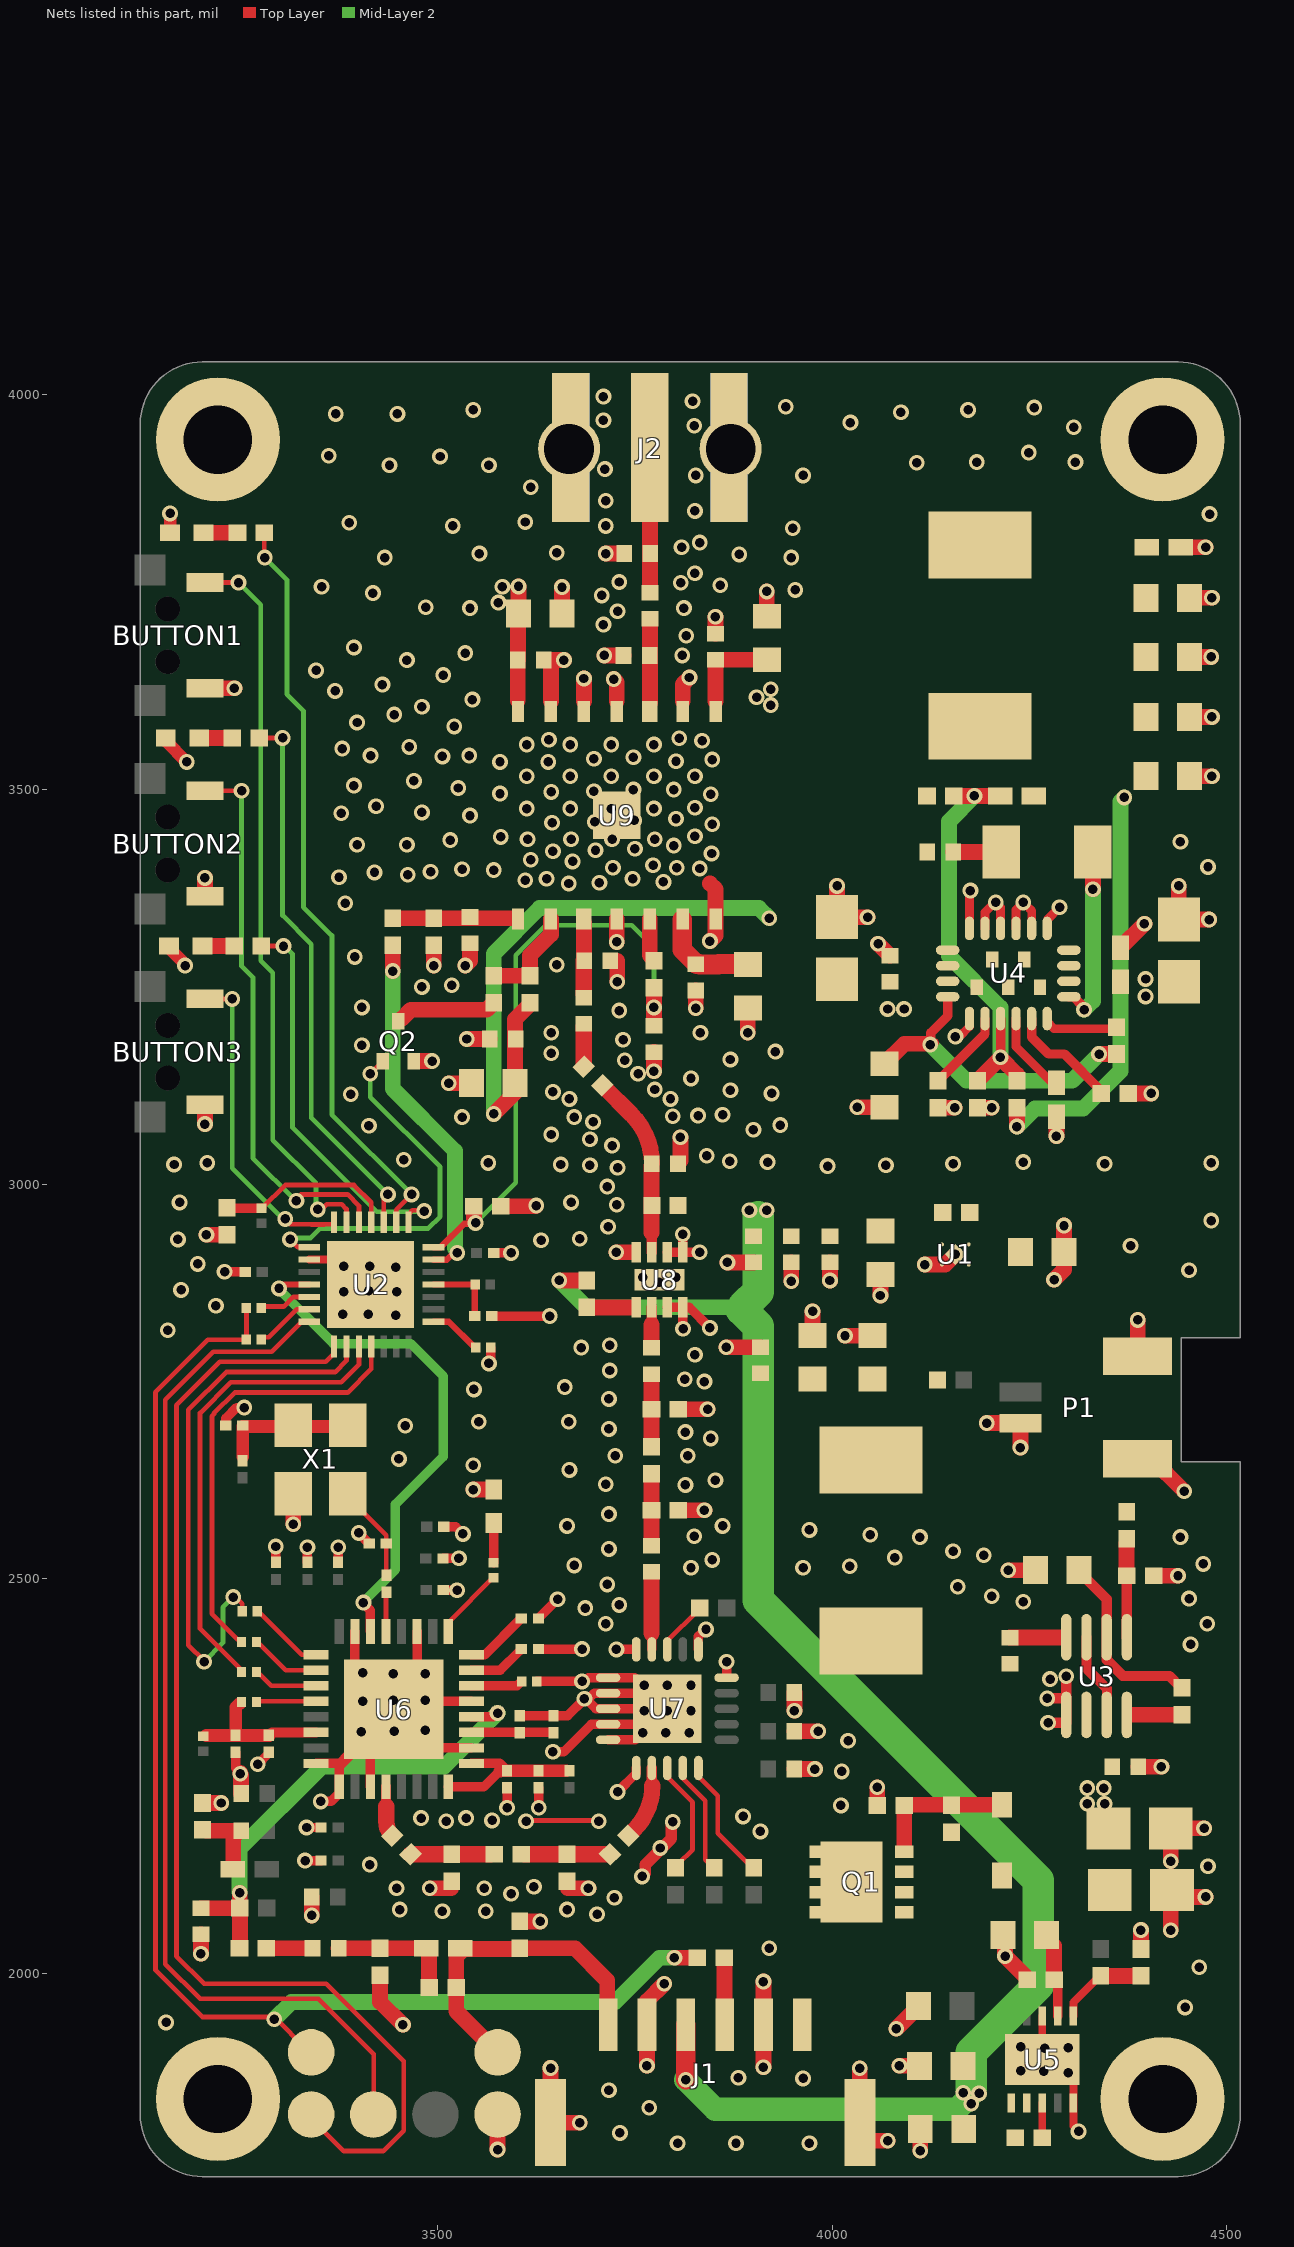
[diagram p0: the nets of this part, all layers, seen from the top]
# Altium PCB MISC79034.PcbDoc (part 2 of 2)
Units mil, origin at the board's own origin, x right, y up, seen from the top; angles counter-clockwise.
Board outline 1393.7 x 2299.21 mil, 4 copper layers (Top Layer, Mid-Layer 1, Mid-Layer 2, Bottom Layer); 179 components, 97 nets, 521 pads, 554 vias.

## Via types
v1: diameter 20, hole 12, Top Layer to Bottom Layer, tented both sides, 554 vias

## Nets (pads, with @x,y where several pads share a name; then routed paths per layer and width w, separated by ;. In a path a pad name is that pad's centre, name@x,y a point inside that pad or via, vN(x,y) a via of type N, cw(c..) or ccw(c..) an arc to the next point about the centre after c; other vN are vias at no path point) (continued)
GND: BUTTON1.1 BUTTON2.1 BUTTON3.1 C1.2 C2.2 C3.2 C4.2 C5.1 C7.1 C8.2 C9.2 C10.2 C11.2 C12.2 C13.2 C14.2 C15.2 C16.2 C17.2 C18.2 C19.1 C20.2 C21.2 C22.1 C23.1 C24.1 C25.1 C26.2 C28.1 C29.2 C30.2 C31.1 C32.1 C33.1 C34.1 C35.2 C36.2 C37.1 C38.2 C39.1 C47.2 C50.2 C51.1 C52.2 C53.1 C54.2 C55.2 C56.1 C57.1 C58.1 C59.1 C60.1 C61.1 C62.1 C63.1 C64.2 C65.2 C67.2 C68.1 C70.1 C71.1 C72.1 C73.2 C74.2 C75.2 C76.2 C78.2 C80.1 C82.2 C83.2 C84.2 J1.2 J1.5 J1.7 J1.8 J2.2 LED1.2 LED2.2 LED3.2 LED4.2 P1.1 P1.3 P1.4 P2.1 Q2.2 R3.1 R6.1 R13.2 R14.2 R15.2 R21.2 R25.1 R29.2 R31.2 R32.2 R33.2 R45.2 R51.2 R52.2 R53.2 R56.2 R57.1 SCREW1.1 SCREW2.1 SCREW3.1 SCREW4.1 SR1.2 U1.2 U1.5 U2.16 U2.29 U3.5 U4.1 U4.11 U4.12 U4.13 U4.14 U4.15 U4.16 U5.5 U5.8 U5.11 U6.8 U6.9 U6.11 U6.18 U6.21 U6.27 U6.31 U6.33 U7.1 U7.10 U7.11 U7.15 U7.16 U7.17 U7.18 U7.19 U7.20 U7.21 U8.3 U8.4 U8.5 U8.6 U8.8 U8.9 U9.4 U9.7 U9.9 U9.11 U9.12 U9.13 U9.15 X1.2 | length 5669
  Top Layer w6: v1@3614,2194 v1@3704,2194
  Top Layer w10: U2.16@3337.26,2904.5 U2.29@3363.5,2904.5 ; U5.11@4266,1921 U5.8@4266,1946.12 ; U5.11@4305.4,1860.4 U5.5@4305.4,1835.88 4305.4,1806.6 v1(4312,1800)
  Top Layer w11: v1(4156,3187) 4161,3187 4173.79,3199.79 U4.1@4173.79,3209.91 ; U4.16@4173.79,3324.09 4173.79,3372 v1(4175,3372) ; U4.15@4193.47,3324.09 4193.47,3344.47 v1@4202,3353 ; v1(4207,3357) 4213.16,3350.84 U4.14@4213.16,3324.09 ; U4.13@4232.84,3324.09 4232.84,3347.84 v1(4242,3357) ; v1@4246,3353 4252.53,3346.47 U4.12@4252.53,3324.09 ; U4.11@4272.21,3324.09 4272.21,3335.21 v1(4288,3351)
  Top Layer w12: v1(3230,2889) C14.2@3256.4,2889 ; C51.1@3231.55,2694.31 3231.55,2703.31 3245.24,2717 v1(3255,2717) ; C68.1@3244,2280.2 3244,2260 v1@3250,2254 ; v1(3272,2265) 3286,2279 C67.2@3286,2280.2 ; C58.1@3295,2520.8 v1(3295,2541) ; v1(3332,2143) C53.1@3352.2,2143 ; v1(3334,2185) C52.2@3352.2,2185 ; C63.1@3335,2520.8 v1(3335,2540) ; U6.8@3346,2266.1 3376.1,2266.1 U6.33@3386,2276 ; v1(3352,2218) 3365,2218 3375.52,2228.52 U6.9@3375.52,2236.58 3375.52,2262.52 3393,2280 U6.33@3398,2280 ; C64.2@3374,2520.8 v1(3374,2540) ; U6.33@3395.21,2390.21 U6.31@3395.21,2433.42 ; v1(3400,2558.2) C47.2@3413.2,2545 ; U6.11@3414.89,2236.58 U6.33@3414.89,2274.89 ; U6.33@3473.95,2391.95 U6.27@3473.95,2433.42 ; U6.33@3503.16,2344.84 U6.21@3542.84,2344.84 ; U6.33@3504.21,2285.79 U6.18@3542.84,2285.79 ; C37.1@3506.8,2526 v1(3527,2526) ; C38.2@3507.26,2485.62 v1(3524.62,2485.62) ; C39.1@3507.8,2566 3523,2566 v1(3532,2557) ; v1(3565,2773) 3567.51,2775.51 R6.1@3567.51,2793 ; C7.1@3568.8,2833 v1(3642,2833) ; C16.2@3570.8,2913 v1(3593,2913) ; v1(3588,2210) C36.2@3588,2235.2 ; C30.2@3604,2326.8 C28.1@3647,2326.8 3664.8,2326.8 v1(3686,2348) ; R25.1@3625.51,2370 v1(3683,2370) ; C29.2@3627.8,2411 v1(3683,2411) ; C32.1@3627.8,2450 v1(3652,2474.2) ; v1(3628,2210) C34.1@3628,2235.2 ; v1(3646,2281) 3660,2281 3694.78,2315.78 U7.19@3715.9,2315.78 U7.21@3749.78,2315.78 ; v1@3687,2371 3690.83,2374.83 U7.16@3715.9,2374.83 3749.83,2374.83 U7.21@3750,2375 ; v1@3691,2345 3700.54,2335.46 U7.18@3715.9,2335.46 U7.21@3750.54,2335.46 ; v1@3693,2350 3698.15,2355.15 U7.17@3715.9,2355.15 U7.21@3750.15,2355.15 ; U7.20@3715.9,2296.09 U7.21@3750.09,2296.09 ; v1(3726.44,2410.56) U7.15@3749,2410.56 ; v1(3728,2230) 3751.63,2253.63 U7.1@3751.63,2260.36 ; U8.3@3790.84,2844.16 3818.84,2844.16 v1(3845,2818) ; U8.6@3790.84,2913.84 v1(3831.84,2913.84) ; U8.4@3810.53,2844.16 3810.53,2817.47 v1(3811,2817) ; U8.5@3810.53,2913.84 v1(3810.53,2936.53) ; U7.11@3830.37,2410.56 3830.37,2427.37 3840,2437 v1(3840,2436) ; U7.10@3866.1,2376 v1(3866.1,2394.9)
  Top Layer w13: v1(4272.41,2348.59) 4296.41,2348.59 U3.5@4296.41,2327.58 ; v1(4273.41,2317.59) 4296.41,2317.59 U3.5@4296.41,2327.58 ; v1(4296.41,2376.59) U3.5@4296.41,2327.58
  Top Layer w15: v1(3759,2123) 3763,2127 3763,2138 3796,2171 v1@3796,2189
  Top Layer w16: LED1.2@3155.61,3565.47 3155.61,3561.39 v1(3182,3535) ; LED3.2@3159.55,3301.69 3159.55,3299.45 3181,3278 v1(3180,3277) ; LED2.2@3161.05,3825.31 v1(3161.05,3849.95)
  Top Layer w20: v1(3200,2025) C80.1@3200,2049.46 ; R53.2@3202,2216.04 v1(3225.96,2216.04) ; v1(3205.14,3076.14) BUTTON3.1@3205.14,3100.9 ; BUTTON2.1@3205.14,3364.68 v1(3205.14,3388.14) ; BUTTON1.1@3205.14,3628.46 v1(3242.54,3628.46) ; v1(3207.04,2935.96) SR1.2@3233,2935.96 ; v1(3250,2253) v1@3250,2254 ; C78.2@3250.88,2228 v1@3250.88,2250.88 ; v1(3317.1,2569.1) X1.2@3317.1,2608 ; v1(3340.46,2073.54) C59.1@3340.46,2097 ; R51.2@3427,1997.96 3427,1964 v1(3456,1935) ; Q2.2@3475,3156 v1@3492,3156 ; v1(3490.04,2107.96) R31.2@3517,2107.96 ; v1(3495,3277) R45.2@3495,3302.96 ; v1(3514,3128) C56.1@3542.9,3128 ; v1(3535,3277) 3541,3283 C5.1@3541,3304.46 ; v1(3537,3184) C57.1@3565.92,3184 ; v1(3545.19,2613.19) LED4.2@3571,2613.19 ; v1(3575.94,1776.94) P2.1@3575.94,1821.38 ; R21.2@3580.04,2972 v1@3624,2972 ; R52.2@3604,2066.04 v1(3629.96,2066.04) ; C54.2@3634.54,3664 v1(3660,3664) ; v1(3643.12,1880.12) J1.8@3643.12,1810.98 v1(3679.98,1810.98) ; U9.13@3643.54,3611.8 C54.2@3643.54,3658.46 ; C55.2@3657.56,3723 v1(3657.56,3756.56) ; R32.2@3665,2107.96 v1(3691.04,2107.96) ; U9.12@3685.27,3611.8 v1(3685.27,3640.73) ; v1(3711,3670) C71.1@3735.46,3670 ; v1(3713,3799) C72.1@3736.46,3799 ; v1(3723,3640) 3727,3636 U9.11@3727,3611.8 ; v1(3726.16,2913.84) U8.8@3746,2913.84 ; v1(3727,3307) U9.4@3727,3336.2 ; v1(3727.54,3256.54) C65.2@3727.54,3283 ; v1(3765.16,1883.16) J1.2@3765.16,1935 3765.16,1965.16 v1(3787,1987) ; v1(3774,3143) C70.1@3774,3167.46 ; C50.2@3807.54,3030 v1(3807.54,3059.54) ; U9.9@3810.46,3611.8 3810.46,3633.46 v1(3819,3642) ; R29.2@3813.04,2587 v1(3838,2587) ; R33.2@3814.04,2715 v1(3842,2715) ; v1(3827,3223) C74.2@3827,3245.46 ; v1(3845,3308) 3852.2,3315.2 U9.7@3852.2,3336.2 3852.2,3373.8 3845,3381 ; C76.2@3852,3697.54 v1(3852,3719) ; v1(3865.54,2793.54) C13.2@3909,2793.54 ; v1(3867.08,2900.92) C33.1@3900,2900.92 ; v1(3893,3192) C73.2@3893,3223.44 ; v1(3912.81,1881.19) J1.5@3912.81,1935 v1(3912.81,1989.81) ; C75.2@3917,3719.56 v1(3917,3751) ; v1(3948,2877) C31.1@3948,2900.92 ; C61.1@3952,2259 v1(3978,2259) ; C60.1@3952,2307 v1(3982,2307) ; v1(3952,2333) C62.1@3952,2356 ; C12.2@3975,2808.56 v1(3975,2839) ; v1(3997,2878) C35.2@3997,2900.92 ; v1(4006,3378) C2.2@4006,3338.37 v1(4044.63,3338.37) ; v1(4016.12,2808.12) C11.2@4051,2808.12 ; v1(4031.56,3097.44) C84.2@4066,3097.44 ; v1(4034.85,1879.85) J1.7@4034.85,1810.98 4034.85,1788.15 v1(4070.15,1788.15) ; R3.1@4056.96,2213 v1(4056.96,2235.96) ; v1(4058,3304.54) C17.2@4073,3289.54 ; v1(4061,2859) C3.2@4061,2885.44 ; v1(4081,1930) 4109.44,1958.44 C24.1@4109.44,1959 ; v1(4085,1883) C26.2@4110.44,1883 ; v1(4111.44,1775.56) C23.1@4111.44,1803 ; v1(4117.2,2898.2) U1.2@4139.07,2898.2 4143.2,2898.2 U1.5@4154,2909 ; R13.2@4134,3096.96 v1(4154.96,3096.96) ; R14.2@4184,3096.92 v1(4201.92,3096.92) ; v1(4195.64,2697.36) P1.1@4238.35,2697.36 v1(4238.35,2666.35) ; C25.1@4216.44,2049 4219,2046.44 v1(4219,2022) 4246.96,1994.04 R57.1@4246.96,1992 ; v1(4223,2511) C1.2@4257.44,2511 ; v1(4281,2879) 4293.56,2891.56 C4.2@4293.56,2914 v1(4293.56,2947.56) ; v1(4284,3061) C22.1@4284,3085.54 ; C18.2@4365,3299.46 v1(4395.54,3330) ; P1.4@4386.97,2652.09 4404.91,2652.09 v1@4445,2612 ; P1.3@4386.97,2782.01 v1(4387,2828) ; C8.2@4387.91,2262 v1(4417,2262) ; R56.2@4391,2031.04 v1(4391,2055) ; R15.2@4407.04,2504 v1(4438,2504) ; v1(4428.74,2054.74) 4428.74,2097 v1(4473,2097) ; v1(4428.74,2142.26) C9.2@4428.74,2184 v1(4471,2184) ; v1(4439,3378) C15.2@4439,3335.37 v1(4477.37,3335.37) ; C19.1@4441.46,3807 v1(4473,3807) ; C21.2@4452.56,3517 v1(4481,3517) ; C83.2@4452.56,3592 v1(4481,3592) ; C20.2@4452.56,3668 v1(4480,3668) ; C82.2@4452.56,3743 v1(4481,3743)
  other v1: 3804,1785 3878,1785 3971,1785 3731,1798 3768,1830 3717,1852 3963,1867 3881,1868 4299,1874 4268,1876 4239,1877 4269,1905 4299,1906 4239,1907 3156,1938 4447,1957 4465,2008 3920,2032 3702,2075 3506,2079 3561,2079 3452,2081 3664,2081 3724,2096 3593,2101 3448,2108 3559,2108 3622,2110 4476,2136 3414,2138 3782,2159 3909,2180 3798,2192 3511,2193 3612,2193 3704,2193 3569,2194 3479,2197 3536,2197 3887,2199 4011,2213 4012,2256 4020,2295 3760,2305 3789,2305 3819,2305 3403,2306 3445,2307 3484,2308 3762,2333 3791,2333 3821,2333 3405,2345 3444,2346 3484,2346 3762,2365 3791,2365 3821,2365 4276,2373 3444,2380 3484,2380 3405,2381 4454,2417 3713,2443 4475,2443 3687,2463 3730,2467 4242,2471 4452,2475 4202,2478 4159,2490 3715,2493 3821,2514 3963,2514 4022,2516 3673,2517 4470,2519 3848,2524 4079,2527 4192,2530 4153,2535 3717,2538 4111,2553 4441,2553 3825,2554 4048,2556 3971,2562 3664,2567 3861,2567 3717,2582 4446,2611 3814,2619 3713,2620 3852,2625 3667,2638 3545,2644 3451,2652 3725,2656 3817,2656 3846,2678 3814,2686 3717,2690 3459,2694 3552,2699 3666,2699 3717,2728 3546,2740 3661,2743 3838,2750 3813,2753 3718,2764 3826,2784 3682,2793 3718,2796 3158,2815 3447,2834 3380,2835 3412,2835 3219,2846 3381,2864 3448,2864 3413,2865 3175,2866 3781,2876 3760,2882 3802,2882 4452,2891 3447,2895 3381,2896 3414,2896 3196,2899 4156,2911 4378,2922 3631,2929 3171,2930 3680,2931 3716,2946 4480,2954 3625,2973 3727,2974 3173,2977 3669,2977 3715,2997 3728,3021 3994,3023 3693,3024 4068,3024 3166,3025 3656,3025 4153,3026 4345,3026 3208,3027 3564,3027 4480,3027 3918,3028 4242,3028 3870,3029 3457,3031 3841,3036 3721,3049 3693,3057 3644,3063 3900,3069 3413,3074 3934,3075 3697,3079 3531,3085 3673,3085 3798,3086 3830,3087 3861,3088 3667,3108 3795,3108 3390,3114 3923,3115 3646,3117 3871,3119 3775,3120 3821,3134 3754,3140 3493,3156 3737,3157 3871,3158 3644,3166 3928,3168 3404,3176 3735,3183 3644,3192 3833,3192 3730,3220 3404,3224 3480,3250 3518,3252 3651,3278 3395,3288 3383,3356 3666,3381 3705,3382 3786,3383 3611,3385 3638,3387 3747,3387 3375,3389 3462,3392 3420,3395 3491,3396 3571,3398 3531,3399 3832,3400 3722,3401 3803,3401 4476,3402 3773,3404 3671,3409 3618,3411 3847,3419 3646,3422 3700,3423 3750,3425 3799,3429 3398,3430 3461,3430 4441,3434 3516,3436 3614,3437 3669,3437 3721,3437 3775,3437 3580,3440 3826,3441 3848,3456 3645,3458 3699,3459 3749,3461 3802,3463 3541,3467 3378,3470 3480,3471 3613,3476 3668,3476 3720,3476 3774,3476 3826,3477 3422,3479 3846,3494 3579,3495 3644,3497 3698,3498 3748,3500 3799,3500 3526,3502 3394,3505 3470,3511 3613,3517 3668,3517 3720,3517 3774,3517 3826,3517 3579,3535 3640,3535 3802,3536 3848,3538 3698,3539 3748,3541 3506,3542 3415,3543 3540,3543 3379,3552 3464,3554 3613,3557 3668,3557 3720,3557 3774,3557 3835,3562 3641,3563 3806,3565 3521,3580 3398,3585 3445,3595 3480,3605 3544,3614 3370,3625 3430,3633 3507,3645 3346,3651 3461,3664 3810,3670 3535,3673 3394,3680 3815,3695 3710,3709 3728,3726 3541,3730 3812,3730 3485,3731 3708,3746 3418,3749 3953,3753 3353,3757 3858,3759 3808,3762 3730,3763 3826,3774 3433,3794 3948,3794 3882,3798 3553,3799 3651,3800 3809,3807 3832,3813 3950,3831 3519,3834 3713,3834 3388,3838 3611,3839 4478,3849 3826,3853 3713,3866 3618,3883 3827,3898 3963,3898 3712,3906 3439,3911 3565,3911 4107,3914 4183,3915 4308,3915 3503,3922 3362,3923 4249,3927 4306,3959 3825,3961 4023,3965 3710,3968 3371,3976 3449,3976 4087,3978 3545,3981 4172,3981 4256,3984 3941,3985 3823,3992 3710,3998
I_RC: P6.1 R4.2 R7.2 R8.2 | length 1715.7
  Top Layer w6: R7.2@3257.49,2803 3209,2803 3142.5,2736.5 3142.5,2404.5 3142.5,2004.5 3202,1945 3293,1945 P6.1@3335,1903 ; R7.2@3257.69,2804.69 R8.2@3257.69,2843
  Top Layer w20: v1(3800,2020) R4.2@3828.96,2020
  Mid-Layer 2 w20: v1(3293,1942) 3315,1964 3725,1964 3781,2020 v1(3800,2020)
LED1: R22.1 U2.10 | length 698.1
  Top Layer w6: R22.1@3273.84,3565.47 v1(3303.53,3565.47) ; U2.10@3431.75,2951.74 3431.75,2981.75 v1(3437,2987)
  Mid-Layer 2 w6: v1(3303.53,3565.47) 3303.53,3340.47 3340,3304 3340,3084 v1@3435,2989
LED2: R2.1 U2.9 | length 954.2
  Top Layer w6: v1@3280.47,3798.53 R2.1@3280.47,3825.31 ; U2.9@3447.5,2951.74 3447.5,2967.5 v1(3467,2987)
  Mid-Layer 2 w6: v1(3281,3794) 3309,3766 3309,3621 3330,3600 3330,3351 3366,3315 3366,3088 v1(3467,2987)
LED3: R23.1 U2.8 | length 496.6
  Top Layer w6: R23.1@3276.59,3301.69 v1(3304.69,3301.69) ; U2.8@3463.24,2951.74 3463.24,2962.24 3468,2967 v1@3479,2967
  Mid-Layer 2 w6: v1@3309,3299 3316,3292 3316,3072 3423,2965 v1@3482,2965
  other v1: 3483,2966
MUXOUT: U2.18 U6.30 | length 653.2
  Top Layer w8: v1@3304,2873 U2.18@3337.26,2873
  Top Layer w12: v1@3407,2468 3414.89,2460.11 U6.30@3414.89,2433.42
  Mid-Layer 2 w12: v1@3298.5,2867.5 3368,2798 3466,2798 3507,2757 3507,2655 3446.5,2594.5 3446.5,2511.5 v1@3407,2472 ; v1@3407,2470 v1@3408,2471
  other v1: 3406,2470 3299,2868
NetC1_1: C1.1 R5.1 U3.2 | length 230.8
  Top Layer w13: C1.1@4315,2507 4347.6,2474.4 U3.2@4347.6,2426 4347.6,2397.4 4368,2377 4427,2377 R5.1@4441,2363
NetC5_2: C5.2 R38.2 R45.1 U9.1 | length 154
  Top Layer w20: R38.2@3443,3337.04 R45.1@3495,3337.04 3572,3337.04 U9.1@3596.96,3337.04
NetC6_1: C6.1 U3.4 | length 66.5
  Top Layer w20: C6.1@4225,2425.54 U3.4@4291.46,2425.54
NetC6_2: C6.2 L2.1 U3.6
NetC7_2: C7.2 R11.1 U2.4 | length 91
  Top Layer w8: U2.4@3494.74,2872.96 R11.1@3546.96,2872.96 ; C7.2@3547.2,2833 R11.1@3547.2,2871.8
NetC22_2: C22.2 U4.4 | length 104.9
  Top Layer w11: U4.4@4232.84,3209.91 4232.84,3174.16 4281,3126 C22.2@4281,3125
NetC25_2: C25.2 R57.2 U5.7 | length 88.8
  Top Layer w12: U5.7@4285.7,1946.12 R57.2@4285.7,1987.7
  Top Layer w20: C25.2@4278,2038 4281.04,2034.96 R57.2@4281.04,1992
NetC27_2: C27.2 C77.1 R50.1 R51.1 | length 157.7
  Top Layer w20: C77.1@3374.54,2032 C27.2@3488,2032 ; R50.1@3489.17,1988.17 C27.2@3489.17,2032.41
NetC28_2: C28.2 C30.1 U6.19 | length 103.7
  Top Layer w12: U6.19@3542.84,2305.47 C28.2@3646.53,2305.47
NetC29_1: C29.1 U6.23 | length 71.4
  Top Layer w12: U6.23@3542.84,2384.21 3579.21,2384.21 C29.1@3604,2409
NetC32_2: C32.2 U6.24 | length 80.8
  Top Layer w12: U6.24@3542.84,2403.9 3559.9,2403.9 C32.2@3605,2449
NetC34_2: C34.2 C36.1 L26.2 U6.16 U6.17 | length 204
  Top Layer w12: U6.16@3513.32,2236.58 3558.58,2236.58 3578.73,2256.73 ; U6.17@3542.84,2266.1 3578.9,2266.1 C36.1@3586,2259
  Top Layer w16: 3579,2256.45 3579.35,2256.8 C36.1@3588,2256.8 C34.2@3628,2256.8 L26.2@3663,2256.8
NetC41_1: C41.1 U6.29 | length 48
  Top Layer w6: U6.29@3434.58,2433.42 C41.1@3434.58,2481.42
NetC41_2: C41.2 C47.1 X1.3 | length 96.8
  Top Layer w6: X1.3@3402,2588 3434.8,2555.2 C47.1@3434.8,2545 ; C41.2@3435,2504.8 C47.1@3435,2545
NetC42_1: C42.1 U6.12 | length 96.5
  Top Layer w13: 3434.58,2217.58 U6.12@3434.58,2236.58
  Top Layer w20.56: 3435,2211.5 3435,2192.33 ccw(c3459.94,2192.33) C42.1@3442.3,2174.7 ; C42.1@3442.3,2174.7 cw(c3459.74,2192.13) 3435.08,2192.13 ccw(c3459.74,2192.13) C42.1@3442.3,2174.7
NetC42_2: C42.2 R30.1 R31.1 | length 101
  Top Layer w20.56: C42.2@3466,2151 R30.1@3567,2151
NetC43_1: C43.1 R30.2 R32.1 | length 105.9
  Top Layer w20.56: R30.2@3610.09,2151 C43.1@3716,2151
NetC43_2: C43.2 U7.2 | length 81.6
  Top Layer w13: 3771.32,2241.36 U7.2@3771.32,2260.36
  Top Layer w20.56: 3748.67,2181.67 ccw(c3692.33,2238) 3772,2238
NetC44_1: C44.1 U7.14 | length 90
  Top Layer w12: U7.14@3771.32,2410.56 3771.32,2429.56
  Top Layer w20.56: 3771,2431 C44.1@3771,2502
NetC44_2: C44.2 R27.1 R29.1 | length 84
  Top Layer w20.56: C44.2@3771,2547 R27.1@3771,2631
NetC45_1: C45.1 R27.2 R33.1 | length 84
  Top Layer w20.56: R27.2@3771,2672 C45.1@3771,2756
NetC45_2: C45.2 U8.2 | length 44
  Top Layer w13: 3771.16,2825.16 U8.2@3771.16,2844.16
  Top Layer w20.56: C45.2@3771,2797 3771,2822
NetC46_1: C46.1 C50.1 L4.1 U8.7 | length 289.9
  Top Layer w13: U8.7@3771.16,2913.84 3771.16,2930.84
  Top Layer w20.56: C46.1@3710,3124 3745.62,3088.38 ; 3771,2939 C50.1@3771,3023 ; 3745.62,3088.38 cw(c3683.24,3026) C50.1@3771.46,3026 ccw(c3683.24,3026) 3745.62,3088.38
NetC46_2: C46.2 C66.2 | length 49.8
  Top Layer w20.56: C46.2@3685,3150.24 3685,3181 C66.2@3685,3200
NetC51_2: C51.2 R39.2 X1.1 X1.4 | length 157
  Top Layer w16: R39.2@3253,2655 3253,2693 X1.4@3372,2693
NetC65_1: C65.1 C66.1 U9.3 | length 90
  Top Layer w20.56: C66.1@3685,3241 U9.3@3685.27,3331
NetC67_1: C67.1 C68.2 R43.2 R47.1 U6.6 | length 182.2
  Top Layer w13: C67.1@3287,2302 3290.47,2305.47 U6.6@3346,2305.47
  Top Layer w16: R47.1@3207,2301.51 C67.1@3286.51,2301.51 ; C68.2@3244,2301.8 3244,2337 R43.2@3249,2342
NetC69_1: C69.1 C71.2 U9.10 | length 104
  Top Layer w20.56: U9.10@3769,3610 C69.1@3769,3714
NetC69_2: C69.2 C72.2 J2.1 | length 175.6
  Top Layer w20.56: C69.2@3769,3757 J2.1@3769,3932.58
NetC77_2: C77.2 R55.2 | length 52.5
  Top Layer w20: R55.2@3283.46,2032 C77.2@3336,2032
NetC79_1: C79.1 C81.1 R53.1 | length 93.3
  Top Layer w20: R53.1@3207,2181 3249,2181 3240.96,2172.96 C81.1@3240.96,2133
NetC84_1: C84.1 R12.2 U4.20 | length 405.2
  Top Layer w12: v1@4122,3176 4125,3176 4126,3176 v1@4129,3179 ; v1@4125,3183 4125,3192 4146.23,3213.23 U4.20@4146.23,3237.47
  Top Layer w20: C84.1@4066,3152.56 4091.44,3178 v1@4122,3178 ; v1(4338.04,3164.96) R12.2@4358,3165
  Mid-Layer 2 w20: v1(4124,3177) 4170,3131 4304.08,3131 v1(4338.04,3164.96)
NetC85_1: C85.1 R54.1 | length 46.5
  Top Layer w20: C85.1@4153.54,3421 R54.1@4200,3421
NetC85_2: C85.2 L3.1 R17.1 U4.9 U4.10 U4.17 U4.18 U4.24 U4.25
NetC86_2: C86.2 R14.1 R16.2 R17.2 U4.3 | length 543.2
  Top Layer w11: v1(4213,3161) v1@4213.16,3161.16
  Top Layer w12: v1@4213.16,3161.16 U4.3@4213.16,3209.91
  Top Layer w20: R17.2@4154.04,3492 v1(4180,3492) C86.2@4204,3492 ; R14.1@4184,3131 v1@4210,3157 ; v1@4214,3159 4234,3139 R16.2@4234,3131
  Mid-Layer 2 w20: v1(4180,3492) 4148,3460 4148,3289 4213,3224 v1(4213,3161)
NetJ1_4: J1.4 R4.1 | length 78.4
  Top Layer w20: J1.4@3863.59,1935 R4.1@3863.59,2013.41
NetJ1_6: J1.6 Q1.5 Q1.6 Q1.7 Q1.8 Q1.9
NetLED1_1: LED1.1 R22.2 | length 34.5
  Top Layer w20: LED1.1@3197.99,3565.47 R22.2@3232.53,3565.47
NetLED2_1: LED2.1 R2.2 | length 38.9
  Top Layer w20: LED2.1@3203.43,3825.31 R2.2@3242.31,3825.31
NetLED3_1: LED3.1 R23.2 | length 35.4
  Top Layer w20: LED3.1@3201.93,3301.69 R23.2@3237.31,3301.69
NetLED4_1: LED4.1 R28.1 | length 42.5
  Top Layer w12: R28.1@3571,2520.51 LED4.1@3571,2563
NetQ1_4: Q1.4 R1.1 R3.2 ZD1.1 | length 176.1
  Top Layer w20: Q1.4@4091.04,2159.04 R3.2@4091.04,2213 ; R3.2@4092.88,2213.88 ZD1.1@4215,2213.88
NetQ2_3: Q2.3 R26.2 | length 124.3
  Top Layer w20: Q2.3@3455,3210 3466,3221 3562.04,3221 R26.2@3571,3229.96
NetR5_2: R5.2 U3.8 | length 62
  Top Layer w20: 4381.04,2327.96 R5.2@4443,2327.96
NetR6_2: R6.2 U2.1 | length 64.4
  Top Layer w8: U2.1@3494.74,2825.76 3514.24,2825.76 R6.2@3546,2794
NetR7_1: R7.1 U2.20 | length 74
  Top Layer w6: R7.1@3278,2806 3286,2806 3321.5,2841.5 U2.20@3337.26,2841.5
NetR8_1: R8.1 U2.19 | length 62.3
  Top Layer w6: R8.1@3280,2845 3305,2845 3317.26,2857.26 U2.19@3337.26,2857.26
NetR9_1: R9.1 U4.5 | length 142.7
  Top Layer w12: U4.5@4252.53,3209.91 4252.53,3186.47 4274,3165 4294,3165 4342,3117 R9.1@4342,3116
NetR10_2: R10.2 R15.1 U3.1 | length 112.4
  Top Layer w13: U3.1@4373.19,2426 R15.1@4373.19,2502.19
  Top Layer w20: R15.1@4372.8,2508.79 R10.2@4372.8,2545
NetR12_1: R12.1 U4.6 | length 99.6
  Top Layer w11: U4.6@4272.21,3209.91 4272.21,3205.79 4281,3197 R12.1@4364,3197
NetR13_1: R13.1 U4.2 | length 96.5
  Top Layer w12: R13.1@4139,3136 4193.47,3190.47 U4.2@4193.47,3209.91
NetR18_2: R18.2 SR1.1 U2.11 | length 233.4
  Top Layer w6: SR1.1@3230,2972 3232.49,2969.51 SR1.1@3234.49,2969.51 ; R18.2@3277,2970 3278,2970 3307,2999 3394,2999 3416,2977 U2.11@3416,2951.71
  Top Layer w12: SR1.1@3234.49,2969.51 R18.2@3277,2969.51
NetR19_1: R19.1 U5.3 | length 40.9
  Top Layer w10: R19.1@4266,1795 U5.3@4266,1835.88
NetR20_2: R20.2 R56.1 U5.6 | length 107.9
  Top Layer w10: U5.6@4305.4,1946.12 4305.4,1963.4 R20.2@4337,1995
  Top Layer w20: R20.2@4345.04,1996.96 R56.1@4391,1996.96
NetR24_2: R24.2 U8.1 | length 58
  Top Layer w20: R24.2@3689,2843.96 U8.1@3746.96,2843.96
NetR25_2: R25.2 U6.22 | length 64
  Top Layer w12: U6.22@3542.84,2364.53 3600.53,2364.53 R25.2@3605,2369
NetR26_1: R26.1 R46.2 U9.2 | length 120.2
  Top Layer w20: R26.1@3571,3264.04 R46.2@3609.96,3264.04 ; R46.2@3617,3266 3617,3290 3643.54,3316.54 U9.2@3643.54,3336.2
NetR28_2: R28.2 U6.25 | length 93.9
  Top Layer w6: U6.25@3513.32,2433.42 3513.32,2444.32 R28.2@3572,2503
NetR34_1: R34.1 U7.3 | length 142.1
  Top Layer w6: U7.3@3791,2260.36 3791,2249 3823,2217 3823,2157 R34.1@3805,2139
NetR35_1: R35.1 U7.13 | length 66
  Top Layer w6: U7.13@3791,2410.56 3791,2421.43 R35.1@3830,2460.43
NetR36_1: R36.1 U7.4 | length 139.4
  Top Layer w6: U7.4@3810.69,2260.36 3810.69,2247.31 3839,2219 3839,2144 R36.1@3847,2136
NetR37_1: R37.1 U7.5 | length 152
  Top Layer w6: U7.5@3830.37,2260.36 3830.37,2249.63 3855,2225 3855,2178 R37.1@3897,2136
NetR40_1: R40.1 U6.1 | length 95.8
  Top Layer w6: R40.1@3273,2459 3328.1,2403.9 U6.1@3346,2403.9
NetR41_1: R41.1 U6.2 | length 88.8
  Top Layer w6: R41.1@3272,2420 3307.78,2384.22 U6.2@3346,2384.22
NetR42_1: R42.1 U6.3 | length 79.8
  Top Layer w6: R42.1@3273,2381 3289.47,2364.53 U6.3@3346,2364.53
NetR43_1: R43.1 U6.4 | length 71.8
  Top Layer w6: R43.1@3274.16,2344.84 U6.4@3346,2344.84
NetR48_2: R48.2 U9.5 | length 53.4
  Top Layer w20: U9.5@3768.73,3336.2 3768.73,3307 3768.73,3290.27 R48.2@3774,3285
NetR54_2: R54.2 U4.7 | length 227.6
  Top Layer w12: U4.7@4299.77,3237.47 4305.53,3237.47 4317,3226 v1@4317,3225
  Top Layer w20: v1(4330.22,3373.78) R54.2@4330.22,3421
  Mid-Layer 2 w20: v1(4319,3221) 4330.22,3232.22 v1(4330.22,3373.78)
ON/OFF: Q2.1 U2.15 | length 465.1
  Top Layer w6: v1(3313,2930) 3322.76,2920.24 U2.15@3337.26,2920.24 ; v1(3414.71,3140) Q2.1@3430.32,3155.61
  Mid-Layer 2 w6: v1@3317,2932 3339,2932 3351,2944 3488,2944 3503,2959 3503,3022 3414.71,3110.29 v1(3414.71,3140)
PA_5.5V: C19.2 C20.1 C21.1 C54.1 C55.1 C56.2 C57.2 C73.1 C74.1 C75.1 C76.1 C82.1 C83.1 C86.1 L3.2 R16.1 R46.1 U9.6 U9.8 U9.14 | length 1650.9
  Top Layer w20: v1(3571,3089) 3598.02,3116.02 C56.2@3598.02,3128 ; C56.2@3598,3132 3598,3209 R46.1@3617,3228 ; 3601.46,3612.54 C54.1@3601.46,3664 ; C54.1@3601.8,3664 C55.1@3601.8,3715.2 ; C55.1@3602.44,3723 v1(3602.44,3757.44) ; C76.1@3852,3664.46 C75.1@3916.46,3664.46 ; U9.8@3852.2,3611.8 C76.1@3852.2,3662.8 ; v1(4234,3073) R16.1@4234,3096.92
  Top Layer w25: U9.6@3810,3335 3810,3297 3828,3279 3831.7,3279 3832.2,3278.5 3855.8,3278.5 3856.3,3279 C73.1@3894,3279
  Mid-Layer 2 w20: v1(3571,3089) 3571,3292 3629,3350 3907,3350 v1(3920,3337) ; v1(4234,3073) 4257,3096 4318,3096 4365,3143 4365,3485 v1(4370,3490)
  other v1: 3922,3607 3904,3617 3922,3627 3577,3737 3582,3757
POWER-IN: C2.1 C8.1 C9.1 C10.1 C15.1 C17.1 C18.1 Q1.1 Q1.2 Q1.3 R1.2 R9.2 U3.3 U3.7 U4.8 U4.19 U4.21 U4.22 U4.23 ZD1.2 | length 120.7
  Top Layer w13: U3.3@4322,2426 4322,2387 4348,2361 U3.7@4348,2345
  Top Layer w20: R9.2@4375.04,3115 v1(4404,3115)
  other v1: 4323,2215 4345,2215 4323,2235 4344,2235 4070,3222 4091,3222 4397,3238 4397,3260
"SPI LE": R42.2 U2.24 | length 593.3
  Top Layer w6: R42.2@3249,2387 3199,2437 3199,2710 3238,2749 3378,2749 3400.26,2771.26 U2.24@3400.26,2794.26
SPICLK: R40.2 U2.23 | length 690.4
  Top Layer w6: 3184,2485 3184,2488 ; v1(3204,2395) 3204,2396 3184,2416 3184,2488 ; v1@3246,2475 3252.49,2468.51 R40.2@3252.49,2459 ; U2.23@3384.5,2794.26 3384.5,2776.5 3370,2762 3232,2762 3184,2714 3184,2488
  Mid-Layer 2 w6: v1(3204,2395) 3228,2419 3228,2464 v1(3241,2477)
SPIDATA: R41.2 U2.25 | length 552.4
  Top Layer w6: R41.2@3247,2423 3214,2456 3214,2706 3216.55,2708.55 3216.55,2709.52 3243.03,2736 3386,2736 3416,2766 U2.25@3416,2794.27
SW1_BAND: BUTTON1.2 U2.13 | length 946.2
  Top Layer w6: BUTTON1.2@3205.14,3762.32 v1(3247.68,3762.32) ; v1(3348,2968) 3353,2968 3359.52,2974.52 3378.48,2974.52 3384.5,2968.5 U2.13@3384.5,2951.74
  Mid-Layer 2 w6: v1@3249,3761 3276,3734 3276,3283 3291,3268 3291,3056 3346,3001 3346,2967 3352,2967 3352,2968 v1(3348,2968)
SW1_FRE: BUTTON2.2 U2.12 | length 706.8
  Top Layer w6: BUTTON2.2@3205.14,3498.54 v1(3251.54,3498.54) ; v1@3319,2979 3327,2987 3386,2987 3400.26,2972.74 U2.12@3400.26,2951.74 ; v1(3321,2979) v1@3321,2980
  Mid-Layer 2 w6: v1(3251.54,3498.54) 3251.54,3276.46 3266,3262 3266,3244 3266,3240 3266,3033 v1@3320,2979
SW1_POWER: BUTTON3.2 U2.14 | length 412.7
  Top Layer w6: BUTTON3.2@3205.14,3234.76 v1(3239.76,3234.76) ; v1@3310,2952 3312.76,2949.24 3339.89,2949.24 3340.13,2949 3355.87,2949 3356.11,2949.24 3368.76,2949.24 U2.14@3368.76,2951.74
  Mid-Layer 2 w6: v1(3239.76,3234.76) 3239.76,3020.24 3308,2952 3307,2953 v1(3307,2956)
SWCLK: P5.1 U2.22 | length 1489.5
  Top Layer w6: P5.1@3354,1802 3381,1775 3431,1775 3456.99,1800.99 3456.99,1849.01 3457,1889 3359,1987 3204,1987 3169,2022 3169,2720 3224,2775 3358,2775 3368.76,2785.76 U2.22@3368.76,2794.26
SWDIO: P4.1 U2.21 | length 1322.6
  Top Layer w6: U2.21@3337.26,2825.76 3327.76,2825.76 3289.62,2787.62 3215.62,2787.62 3155,2727 3155,2012 3199,1968 3349,1968 3419,1898 3419,1829 P4.1@3416,1826
VCC_5V: C3.1 C23.2 C26.1 C31.2 C33.2 C35.1 J1.3 L4.2 R19.2 R24.1 R44.2 U1.1 U5.1 U5.2 | length 2037.6
  Top Layer w20: v1(3654.04,2878.04) R24.1@3689,2878.04
  Top Layer w25: v1(3814.37,1865.37) J1.3@3814.37,1935
  Mid-Layer 2 w20: v1(3654.04,2878.04) 3688.08,2844 3888,2844
  Mid-Layer 2 w30: v1(3814.37,1865.37) 3851.73,1828 4158,1828 v1@4173,1843
  Mid-Layer 2 w40: 3906,2959 3906,2864 3888,2846 3888,2844 3885,2841 3906,2820 3906,2473 4261,2118 4261,1985 4176,1900 4176,1854
  other v1: 4176,1835 4186,1848 4166,1849 3895,2967 3917,2967
VCC_5V3: C4.1 C11.1 C12.1 C13.1 L1.2 L2.2 R10.1 R44.1 U1.3 U1.4
VDET: C70.2 R21.1 R48.1 U2.7 | length 761.8
  Top Layer w8: U2.7@3494.74,2920.24 3504.24,2920.24 3504.95,2920.95 3504.95,2921.28 3533.66,2950 v1@3548,2950
  Top Layer w20: R21.1@3545.96,2972 3545.96,2957.04 v1@3546,2957 ; C70.2@3774,3205 v1(3774,3224) R48.1@3774,3248.96
  Mid-Layer 2 w6: v1@3549,2952 3599,3002 3599,3290 3637,3328 3746,3328 3774,3300 v1(3774,3224)
  other v1: 3548,2951
VIDEO-IN: C27.1 J1.1 P7.1 R50.2 R52.1 | length 402
  Top Layer w20: P7.1@3570,1906 3523.67,1952.33 R50.2@3523.67,1982.41 3523.67,2021.67 3533,2031 R52.1@3600,2031 ; R52.1@3604,2031.96 3674.04,2031.96 3715,1991 J1.1@3715,1932
VREF: R38.1 U2.6 | length 463.2
  Top Layer w8: U2.6@3494.74,2904.5 3511.5,2904.5 3524,2917 3524.52,2917 3524.95,2916.57 3524.95,2912.72 3525,2912.72 3525,2913 v1(3524.95,2913)
  Top Layer w20: v1(3443,3270) R38.1@3443,3302.96
  Mid-Layer 2 w8: v1@3524.52,2917.48 3524.52,2917 3524.95,2916.57 3524.95,2912.72 3525,2912.72 3525,2913 v1(3524.95,2913)
  Mid-Layer 2 w20: v1(3443,3270) 3443,3121 3522,3042 3522,2919 v1@3523,2918
VTUNE: C80.2 R49.2 R55.1 U6.20 | length 602.9
  Top Layer w12: U6.20@3542.84,2325.16 3571.16,2325.16 v1(3576,2330)
  Top Layer w20: C80.2@3200,2082.54 3249.54,2082.54 3249.54,2057 ; R49.2@3249.38,2083 v1(3249.38,2102.38) ; R55.1@3249.54,2037.46 3249.54,2057 ; 3250,2057 3249.54,2057
  Mid-Layer 2 w20: v1@3249,2103 3249,2158 3353,2262 3508,2262 v1(3576,2330)
pads on no net: BUTTON1.0 BUTTON1.3 BUTTON1.4 BUTTON2.0 BUTTON2.3 BUTTON2.4 BUTTON3.0 BUTTON3.3 BUTTON3.4 U2.2 U2.3 U5.4 U6.5 U6.13 U6.14 U6.15 U6.26 U7.6 U7.7 U7.8 U7.12

## Polygon pours and split planes (outlines as drawn)
PA_5.5V on Top Layer "Bottom Layer-No Net" (solid, remove dead copper): 4239,3498 4239,3481 4239,3477 4241,3475 4244,3472 4253,3472 4399,3472 4407,3480 4414,3487 4414,3514 4414,3809 4361,3862 4340,3883 4212,3883 4027,3883 3986,3842 3981,3837 3981,3787 3981,3710 3953,3682 3951,3680 3931,3680 3899,3680 3895,3676 3894,3675 3874,3675 3846,3675 3844,3673 3842,3671 3842,3659 3842,3589 3844,3587 3845,3586 3852,3586 3871,3586 3878,3579 3891,3566 3891,3484 3891,3313 3878,3300 3874,3296 3874,3281 3874,3265 3876,3263 3883,3263 3937,3263 3949,3275 3956,3282 3956,3326 3956,3406 3969,3419 3996,3446 3996,3536 3996,3605 4022,3631 4111,3720 4239,3720 4286,3720 4304,3702 4321,3685 4321,3657 4321,3532 4312,3523 4301,3512 4274,3512 4243,3512 4241,3510 4239,3508 4239,3499
NetC85_2 on Top Layer "Bottom Layer-No Net" (solid, remove dead copper): 4034,3570 4034,3406 4080,3360 4080,3346 4080,3324 4123,3281 4133,3271 4151,3271 4315,3271 4317,3273 4318,3274 4318,3280 4318,3297 4315,3300 4313,3302 4307,3302 4169,3302 4163,3308 4160,3311 4160,3325 4160,3356 4139,3377 4131,3385 4131,3416 4131,3509 4141,3519 4151,3529 4177,3529 4251,3529 4258,3536 4265,3543 4265,3561 4265,3617 4258,3624 4254,3628 4236,3628 4092,3628 4034,3570
POWER-IN on Top Layer "Bottom Layer-No Net" (solid, remove dead copper): 3971,3263 3971,3210 3984,3197 4097,3197 4104,3197 4111,3204 4116,3209 4116,3224 4116,3238 4123,3245 4129,3251 4138,3251 4167,3251 4170,3248 4171,3247 4171,3242 4171,3237 4173,3235 4175,3233 4180,3233 4271,3233 4274,3236 4276,3238 4276,3241 4276,3244 4280,3248 4283,3251 4292,3251 4332,3251 4337,3246 4338,3245 4338,3239 4338,3233 4342,3229 4347,3224 4379,3224 4467,3224 4472,3229 4474,3231 4474,3238 4474,3276 4468,3282 4465,3285 4457,3285 4397,3285 4386,3274 4385,3273 4360,3273 4334,3273 4330,3269 4325,3264 4302,3264 4124,3264 4121,3267 4120,3268 4112,3268 4064,3268 4050,3282 4044,3288 4008,3288 3981,3288 3974,3281 3971,3278 3971,3265
3.3V on Top Layer "Bottom Layer-No Net" (solid, remove dead copper): 4148,1973 4148,1942 4151,1939 4157,1933 4228,1933 4250,1933 4252,1935 4253,1936 4253,1940 4253,1962 4249,1966 4248,1967 4238,1967 4224,1967 4219,1972 4214,1977 4214,1996 4214,2003 4204,2013 4201,2016 4178,2016 4166,2016 4159,2009 4148,1998 4148,1974
VCC_5V on Top Layer "Bottom Layer-No Net" (solid, remove dead copper): 4149,1866 4149,1779 4152,1776 4161,1767 4175,1767 4234,1767 4240,1773 4242,1775 4242,1784 4242,1807 4251,1816 4252,1817 4252,1826 4252,1847 4251,1848 4250,1849 4242,1849 4210,1849 4206,1853 4197,1862 4197,1882 4197,1897 4191,1903 4190,1904 4171,1904 4154,1904 4151,1901 4149,1899 4149,1865
POWER-IN on Top Layer "Bottom Layer-No Net" (solid, remove dead copper): 4078,2128 4078,2095 4078,2061 4082,2057 4085,2054 4086,2053 4140,2053 4148,2053 4157,2062 4161,2066 4161,2079 4161,2083 4167,2089 4179,2101 4207,2101 4295,2101 4318,2078 4322,2074 4346,2074 4371,2074 4376,2079 4380,2083 4380,2098 4380,2235 4373,2242 4366,2249 4366,2259 4366,2291 4359,2298 4358,2299 4358,2320 4358,2362 4356,2364 4355,2365 4352,2365 4342,2365 4339,2362 4339,2354 4339,2266 4319,2246 4287,2214 4287,2202 4287,2183 4279,2175 4269,2165 4254,2165 4205,2165 4190,2180 4180,2190 4159,2190 4137,2190 4129,2182 4126,2179 4126,2162 4126,2152 4120,2146 4111,2137 4096,2137 4080,2137 4079,2136 4078,2135 4078,2129
PA_5.5V on Top Layer "Bottom Layer-No Net" (solid, remove dead copper, pour order 1001): 3566,3755 3566,3598 3574,3590 3579,3585 3594,3585 3609,3585 3611,3587 3612,3588 3612,3629 3612,3696 3620,3704 3620,3721 3620,3770 3612,3778 3608,3782 3602,3782 3580,3782 3575,3777 3566,3768 3566,3755
GND on Top Layer "Bottom Layer-No Net" (solid, remove dead copper, pour order 1011): 2958.39,3939.39 2964.39,3933.39 2964.39,1959.39 2964.39,1840.39 3024.39,1780.39 3073.39,1731.39 3235.39,1731.39 4521.39,1731.39 4586.39,1796.39 4613.39,1823.39 4613.39,1867.39 4613.39,4069.39 4559.39,4123.39 4439.39,4243.39 4168.39,4243.39 3089.39,4243.39 2975.39,4129.39 2953.39,4107.39 2953.39,3950.39
VCC_5V3 on Top Layer "Bottom Layer-No Net" (solid, remove dead copper, pour order 1004): 4162,2966 4162,2931 4171,2922 4175,2918 4175,2909 4175,2903 4175,2902 4095,2822 4088,2815 4088,2801 4088,2785 4080,2777 4073,2770 3986,2770 3899,2770 3890,2761 3886,2757 3886,2731 3886,2647 3915,2618 3933,2600 4107,2600 4140,2600 4158,2582 4167,2573 4373,2573 4385,2573 4388,2576 4391,2579 4391,2583 4391,2600 4387,2604 4386,2605 4372,2605 4211,2605 4180,2636 4145,2671 4145,2755 4145,2801 4160,2816 4207,2863 4230,2863 4248,2881 4255,2888 4255,2913 4255,2950 4238,2967 4221,2984 4197,2984 4168,2984 4164,2980 4162,2978 4162,2966
VCC_5V on Top Layer "Bottom Layer-No Net" (solid, remove dead copper, pour order 1003): 3804,2975 3804,2956 3805,2955 3807,2953 3817,2953 3867,2953 3873,2947 3878,2942 3878,2935 3878,2930 3882,2926 3884,2924 3895,2924 4086,2924 4091,2919 4132,2919 4139,2919 4142,2922 4150,2930 4150,2956 4150,2980 4146,2984 4142,2988 4129,2988 3808,2988 3807,2987 3804,2984 3804,2975
+5V-FAN on Top Layer "Bottom Layer-No Net" (solid, remove dead copper, pour order 1002): 4155,2757 4155,2733 4159,2729 4164,2724 4214,2724 4263,2724 4267,2728 4270,2731 4270,2733 4270,2767 4266,2771 4262,2775 4248,2775 4165,2775 4156,2766 4155,2765 4155,2758
NetC6_2 on Top Layer "Bottom Layer-No Net" (solid, remove dead copper, pour order 1001): 3975,2442 3975,2366 3981,2360 3987,2354 4019,2354 4051,2354 4067,2338 4076,2329 4076,2305 4076,2283 4109,2250 4117,2242 4206,2242 4297,2242 4316,2261 4332,2277 4332,2329 4332,2356 4328,2360 4324,2360 4317,2360 4314,2357 4312,2355 4312,2346 4312,2296 4304,2288 4301,2285 4293,2285 4261,2285 4251,2295 4248,2298 4248,2371 4248,2397 4244,2401 4243,2402 4235,2402 4198,2402 4174,2426 4124,2476 4094,2476 3992,2476 3983,2467 3975,2459 3975,2443
NetJ1_6 on Top Layer "Bottom Layer-No Net" (solid, remove dead copper, pour order 1000): 3949,1966 3949,1945 3949,1901 3950,1900 3951,1899 3953,1899 4001,1899 4005,1903 4007,1905 4007,1920 4007,1969 4049,2011 4064,2026 4064,2074 4064,2167 4061,2170 4060,2171 4050,2171 3972,2171 3966,2165 3964,2163 3964,2148 3964,2021 3961,2018 3949,2006 3949,1966
POWER-IN on Mid-Layer 2 "Bottom Layer-No Net" (solid, remove dead copper): 3948,3227 3948,2491 4141,2298 4254,2185 4321,2185 4436,2185 4457,2206 4486,2235 4486,2254 4486,2552 4431,2607 4420,2618 4420,2697 4420,2811 4431,2822 4434,2825 4457,2825 4476,2825 4483,2832 4496,2845 4496,2898 4496,3256 4480,3272 4473,3279 4456,3279 4402,3279 4397,3274 4387,3264 4387,3257 4387,3097 4364,3074 4342,3052 4247,3052 4194,3052 4152,3094 4106,3140 4106,3211 4106,3241 4098,3249 4094,3253 4076,3253 3967,3253 3953,3239 3948,3234 3948,3227
PA_5.5V on Mid-Layer 2 "Bottom Layer-No Net" (solid, remove dead copper, pour order 1000): 3567,3767 3567,3757 3567,3627 3606,3588 3614,3580 3627,3580 3926,3580 3935,3589 3937,3591 3937,3596 3937,3637 3932,3642 3931,3643 3928,3643 3907,3643 3901,3637 3887,3623 3818,3623 3660,3623 3629,3654 3620,3663 3620,3693 3620,3767 3612,3775 3610,3777 3603,3777 3576,3777 3569,3770 3567,3768 3567,3767
GND on Mid-Layer 2 "Bottom Layer-No Net" (solid, remove dead copper, pour order 1016): 2935.62,3735.2 2935.62,1800.2 3033.62,1702.2 3058.62,1677.2 3285.62,1677.2 4524.62,1677.2 4608.62,1761.2 4662.62,1815.2 4662.62,2032.2 4662.62,3952.2 4504.62,4110.2 4460.62,4154.2 4341.62,4154.2 3088.62,4154.2 3019.62,4085.2 2930.62,3996.2 2930.62,3759.2
VCC_5V on Mid-Layer 2 "Bottom Layer-No Net" (solid, remove dead copper, pour order 1014): 4165,1820 4186,1820 4195,1820 4199,1824 4204,1829 4204,1834 4204,1854 4202,1856 4197,1861 4167,1861 4154,1861 4151,1858 4149,1856 4149,1847 4149,1825 4151,1823 4154,1820 4164,1820
VCC_5V on Mid-Layer 2 "Bottom Layer-No Net" (solid, remove dead copper, pour order 1013): 3883,2975 3883,2957 3887,2953 3889,2951 3895,2951 3925,2951 3928,2954 3930,2956 3930,2961 3930,2977 3926,2981 3925,2982 3913,2982 3890,2982 3883,2975
3.3V on Mid-Layer 2 "Bottom Layer-No Net" (solid, remove dead copper, pour order 1012): 4153.5,2011 4153.5,1978 4158.5,1973 4164.5,1967 4174.5,1967 4191.5,1967 4197.5,1973 4204.5,1980 4204.5,1987 4204.5,2012 4195.5,2021 4190.5,2026 4188.5,2026 4164.5,2026 4161.5,2023 4153.5,2015 4153.5,2012
GND on Bottom Layer "Bottom Layer-No Net" (solid, remove dead copper, pour order 1017): 2917,3744 2917,1820 3075,1662 3115,1622 3420,1622 4605,1622 4674,1691 4728,1745 4728,1997 4728,3913 4536,4105 4497,4144 4166,4144 3085,4144 2991,4050 2917,3976 2917,3769
GND on Mid-Layer 1 "Bottom Layer-No Net" (solid, remove dead copper, pour order 1018): 3038,3841 3038,1740 3109,1669 3329,1669 4550,1669 4597,1716 4746,1865 4746,2086 4746,3927 4541,4132 4439,4234 4046,4234 3202,4234 3077,4109 3034,4066 3034,3841

## Keep-outs
Keep-Out Layer:
  the board outline again, w3.94

## Other copper
Mid-Layer 1:
  pour cut-out: 3725,3838 3813,3838 3813,4037 3726,4037 3725,4038

## Silkscreen, mask and mechanical layers (free items; w line width, h text height)
Top Overlay:
  lines w3.94: 3123.45,3006.68 3709.8,3006.68 3709.8,3046.7 3124.1,3046.7 ; 4516.63,3006.68 3847.6,3006.68 3847.6,3046.7 4516.89,3046.7
  text "CLK" at 3301,1756 h40
  text "3.3V" at 3463,1756 h40
  text "DIO" at 3391,1755 h40
  text "GND" at 3542,1755 h40
Top Solder:
  rectangle: 3123.19,3006.42 3711.2,3045.79
  rectangle: 3847.6,3002.48 4516.89,3049.72
Bottom Solder:
  region: 1 vertices and 45 holes, not listed, extent -1859,-73 -1859,-73